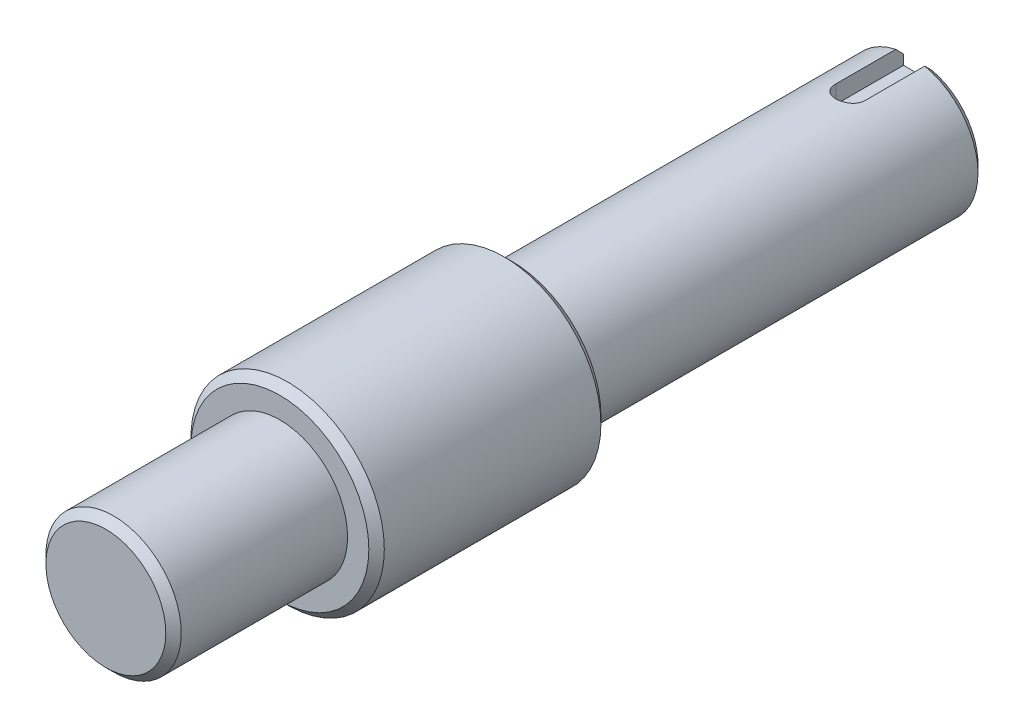
from build123d import *

# Parameters (mm, degrees)
BOSS_EXTRUDE1_DEPTH      = 150
BOSS_EXTRUDE1_DEPTH_BACK = 270
SKETCH1_R                = 35
SKETCH2_R                = 50
BOSS_EXTRUDE2_DEPTH      = 60
CHAMFER1_SIZE            = 4
CUT_EXTRUDE1_DEPTH       = 10


with BuildPart() as part:
    # Sketch1 → Boss-Extrude1 (new, two sides: drawn at the far end of the back side and taken through both)
    with BuildSketch(Plane.XY.offset(-BOSS_EXTRUDE1_DEPTH_BACK)):
        Circle(SKETCH1_R)
    extrude(amount=BOSS_EXTRUDE1_DEPTH + BOSS_EXTRUDE1_DEPTH_BACK)

    # Sketch2 → Boss-Extrude2 (add, symmetric)
    with BuildSketch(Plane.XY):
        Circle(SKETCH2_R)
    extrude(amount=BOSS_EXTRUDE2_DEPTH, both=True)

    # Chamfer1
    chamfer1_edges = [part.edges().sort_by_distance(p)[0] for p in [
        (-35, 0, -270),
        (-35, 0, 150),
        (-50, 0, -60),
        (-50, 0, 60),
    ]]
    chamfer(chamfer1_edges, length=CHAMFER1_SIZE)

    # Sketch3 → Cut-Extrude1 (cut)
    with BuildSketch(Plane(origin=(0, 35, 0), x_dir=(1, 0, 0), z_dir=(0, 1, 0))):
        with BuildLine():
            Line((-7.5, 305), (7.5, 305))
            Line((7.5, 305), (7.5, 235))
            ThreePointArc((7.5, 235), (0, 227.5), (-7.5, 235))
            Line((-7.5, 235), (-7.5, 305))
        make_face()
    extrude(amount=-CUT_EXTRUDE1_DEPTH, mode=Mode.SUBTRACT)


solid = part.part
